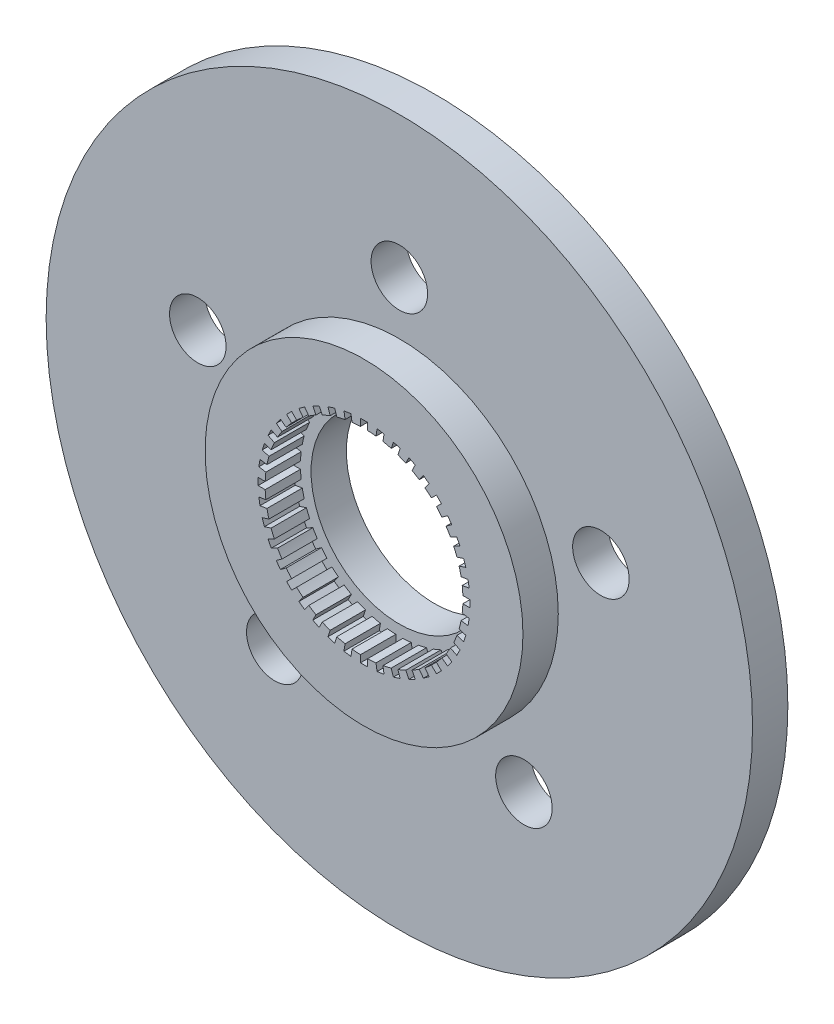
from build123d import *

# Parameters (mm, degrees)
SKETCH_1_R      = 100
SKETCH_1_R_2    = 25
SKETCH_1_R_3    = 8
EXTRUDE_1_DEPTH = 10
EXTRUDE_START   = -10
SKETCH_2_R      = 45
EXTRUDE_2_DEPTH = 20


with BuildPart() as part:
    # 草图1 → 凸台-拉伸1 (new body)
    with BuildSketch(Plane.XY):
        Circle(SKETCH_1_R)
        Circle(SKETCH_1_R_2, mode=Mode.SUBTRACT)
        with Locations((0, 60)):
            Circle(SKETCH_1_R_3, mode=Mode.SUBTRACT)
        with Locations((57.063390978, 18.541019663)):
            Circle(SKETCH_1_R_3, mode=Mode.SUBTRACT)
        with Locations((35.267115138, -48.541019662)):
            Circle(SKETCH_1_R_3, mode=Mode.SUBTRACT)
        with Locations((-35.267115138, -48.541019663)):
            Circle(SKETCH_1_R_3, mode=Mode.SUBTRACT)
        with Locations((-57.063390978, 18.541019662)):
            Circle(SKETCH_1_R_3, mode=Mode.SUBTRACT)
    extrude(amount=EXTRUDE_1_DEPTH)

    # 草图2 → 凸台-拉伸2 (add)
    with BuildSketch(Plane.XY.offset(10).offset(EXTRUDE_START)):
        Circle(SKETCH_2_R)
        with BuildLine():
            Line((3.389682317, 27.794065082), (3.702737645, 29.770618635))
            Line((3.702737645, 29.770618635), (5.678114326, 29.457749705))
            Line((5.678114326, 29.457749705), (5.365058998, 27.481196152))
            ThreePointArc((5.365058998, 27.481196152), (6.536470188, 27.226357771), (7.695899405, 26.92161088))
            Line((7.695899405, 26.92161088), (8.3143016, 28.824857136))
            Line((8.3143016, 28.824857136), (10.216414633, 28.206823147))
            Line((10.216414633, 28.206823147), (9.598012437, 26.303576891))
            ThreePointArc((9.598012437, 26.303576891), (10.715136106, 25.86862691), (11.812617909, 25.386257269))
            Line((11.812617909, 25.386257269), (12.721139857, 27.169331989))
            Line((12.721139857, 27.169331989), (14.503152905, 26.26135099))
            Line((14.503152905, 26.26135099), (13.594630957, 24.47827627))
            ThreePointArc((13.594630957, 24.47827627), (14.629959812, 23.873924602), (15.638470555, 23.225809753))
            Line((15.638470555, 23.225809753), (16.814741431, 24.844807719))
            Line((16.814741431, 24.844807719), (18.43277542, 23.669237215))
            Line((18.43277542, 23.669237215), (17.256504544, 22.050239248))
            ThreePointArc((17.256504544, 22.050239248), (18.184545353, 21.291367037), (19.079252156, 20.493465719))
            Line((19.079252156, 20.493465719), (20.494308266, 21.908521828))
            Line((20.494308266, 21.908521828), (21.908521828, 20.494308266))
            Line((21.908521828, 20.494308266), (20.493465719, 19.079252156))
            ThreePointArc((20.493465719, 19.079252156), (21.291367037, 18.184545353), (22.050239248, 17.256504544))
            Line((22.050239248, 17.256504544), (23.669237215, 18.43277542))
            Line((23.669237215, 18.43277542), (24.844807719, 16.814741431))
            Line((24.844807719, 16.814741431), (23.225809753, 15.638470555))
            ThreePointArc((23.225809753, 15.638470555), (23.873924602, 14.629959812), (24.47827627, 13.594630957))
            Line((24.47827627, 13.594630957), (26.26135099, 14.503152905))
            Line((26.26135099, 14.503152905), (27.169331989, 12.721139857))
            Line((27.169331989, 12.721139857), (25.386257269, 11.812617909))
            ThreePointArc((25.386257269, 11.812617909), (25.86862691, 10.715136106), (26.303576891, 9.598012437))
            Line((26.303576891, 9.598012437), (28.206823147, 10.216414633))
            Line((28.206823147, 10.216414633), (28.824857136, 8.3143016))
            Line((28.824857136, 8.3143016), (26.92161088, 7.695899405))
            ThreePointArc((26.92161088, 7.695899405), (27.226357771, 6.536470188), (27.481196152, 5.365058998))
            Line((27.481196152, 5.365058998), (29.457749705, 5.678114326))
            Line((29.457749705, 5.678114326), (29.770618635, 3.702737645))
            Line((29.770618635, 3.702737645), (27.794065082, 3.389682317))
            ThreePointArc((27.794065082, 3.389682317), (27.913685345, 2.19685468), (27.982137159, 1))
            Line((27.982137159, 1), (29.983328701, 1))
            Line((29.983328701, 1), (29.983328701, -1))
            Line((29.983328701, -1), (27.982137159, -1))
            ThreePointArc((27.982137159, -1), (27.913685345, -2.19685468), (27.794065082, -3.389682317))
            Line((27.794065082, -3.389682317), (29.770618635, -3.702737645))
            Line((29.770618635, -3.702737645), (29.457749705, -5.678114326))
            Line((29.457749705, -5.678114326), (27.481196152, -5.365058998))
            ThreePointArc((27.481196152, -5.365058998), (27.226357771, -6.536470188), (26.92161088, -7.695899405))
            Line((26.92161088, -7.695899405), (28.824857136, -8.3143016))
            Line((28.824857136, -8.3143016), (28.206823147, -10.216414633))
            Line((28.206823147, -10.216414633), (26.303576891, -9.598012437))
            ThreePointArc((26.303576891, -9.598012437), (25.86862691, -10.715136106), (25.386257269, -11.812617909))
            Line((25.386257269, -11.812617909), (27.169331989, -12.721139857))
            Line((27.169331989, -12.721139857), (26.26135099, -14.503152905))
            Line((26.26135099, -14.503152905), (24.47827627, -13.594630957))
            ThreePointArc((24.47827627, -13.594630957), (23.873924602, -14.629959812), (23.225809753, -15.638470555))
            Line((23.225809753, -15.638470555), (24.844807719, -16.814741431))
            Line((24.844807719, -16.814741431), (23.669237215, -18.43277542))
            Line((23.669237215, -18.43277542), (22.050239248, -17.256504544))
            ThreePointArc((22.050239248, -17.256504544), (21.291367037, -18.184545353), (20.493465719, -19.079252156))
            Line((20.493465719, -19.079252156), (21.908521828, -20.494308266))
            Line((21.908521828, -20.494308266), (20.494308266, -21.908521828))
            Line((20.494308266, -21.908521828), (19.079252156, -20.493465719))
            ThreePointArc((19.079252156, -20.493465719), (18.184545353, -21.291367037), (17.256504544, -22.050239248))
            Line((17.256504544, -22.050239248), (18.43277542, -23.669237215))
            Line((18.43277542, -23.669237215), (16.814741431, -24.844807719))
            Line((16.814741431, -24.844807719), (15.638470555, -23.225809753))
            ThreePointArc((15.638470555, -23.225809753), (14.629959812, -23.873924602), (13.594630957, -24.47827627))
            Line((13.594630957, -24.47827627), (14.503152905, -26.26135099))
            Line((14.503152905, -26.26135099), (12.721139857, -27.169331989))
            Line((12.721139857, -27.169331989), (11.812617909, -25.386257269))
            ThreePointArc((11.812617909, -25.386257269), (10.715136106, -25.86862691), (9.598012437, -26.303576891))
            Line((9.598012437, -26.303576891), (10.216414633, -28.206823147))
            Line((10.216414633, -28.206823147), (8.3143016, -28.824857136))
            Line((8.3143016, -28.824857136), (7.695899405, -26.92161088))
            ThreePointArc((7.695899405, -26.92161088), (6.536470188, -27.226357771), (5.365058998, -27.481196152))
            Line((5.365058998, -27.481196152), (5.678114326, -29.457749705))
            Line((5.678114326, -29.457749705), (3.702737645, -29.770618635))
            Line((3.702737645, -29.770618635), (3.389682317, -27.794065082))
            ThreePointArc((3.389682317, -27.794065082), (2.19685468, -27.913685345), (1, -27.982137159))
            Line((1, -27.982137159), (1, -29.983328701))
            Line((1, -29.983328701), (-1, -29.983328701))
            Line((-1, -29.983328701), (-1, -27.982137159))
            ThreePointArc((-1, -27.982137159), (-2.19685468, -27.913685345), (-3.389682317, -27.794065082))
            Line((-3.389682317, -27.794065082), (-3.702737645, -29.770618635))
            Line((-3.702737645, -29.770618635), (-5.678114326, -29.457749705))
            Line((-5.678114326, -29.457749705), (-5.365058998, -27.481196152))
            ThreePointArc((-5.365058998, -27.481196152), (-6.536470188, -27.226357771), (-7.695899405, -26.92161088))
            Line((-7.695899405, -26.92161088), (-8.3143016, -28.824857136))
            Line((-8.3143016, -28.824857136), (-10.216414633, -28.206823147))
            Line((-10.216414633, -28.206823147), (-9.598012437, -26.303576891))
            ThreePointArc((-9.598012437, -26.303576891), (-10.715136106, -25.86862691), (-11.812617909, -25.386257269))
            Line((-11.812617909, -25.386257269), (-12.721139857, -27.169331989))
            Line((-12.721139857, -27.169331989), (-14.503152905, -26.26135099))
            Line((-14.503152905, -26.26135099), (-13.594630957, -24.47827627))
            ThreePointArc((-13.594630957, -24.47827627), (-14.629959812, -23.873924602), (-15.638470555, -23.225809753))
            Line((-15.638470555, -23.225809753), (-16.814741431, -24.844807719))
            Line((-16.814741431, -24.844807719), (-18.43277542, -23.669237215))
            Line((-18.43277542, -23.669237215), (-17.256504544, -22.050239248))
            ThreePointArc((-17.256504544, -22.050239248), (-18.184545353, -21.291367037), (-19.079252156, -20.493465719))
            Line((-19.079252156, -20.493465719), (-20.494308266, -21.908521828))
            Line((-20.494308266, -21.908521828), (-21.908521828, -20.494308266))
            Line((-21.908521828, -20.494308266), (-20.493465719, -19.079252156))
            ThreePointArc((-20.493465719, -19.079252156), (-21.291367037, -18.184545353), (-22.050239248, -17.256504544))
            Line((-22.050239248, -17.256504544), (-23.669237215, -18.43277542))
            Line((-23.669237215, -18.43277542), (-24.844807719, -16.814741431))
            Line((-24.844807719, -16.814741431), (-23.225809753, -15.638470555))
            ThreePointArc((-23.225809753, -15.638470555), (-23.873924602, -14.629959812), (-24.47827627, -13.594630957))
            Line((-24.47827627, -13.594630957), (-26.26135099, -14.503152905))
            Line((-26.26135099, -14.503152905), (-27.169331989, -12.721139857))
            Line((-27.169331989, -12.721139857), (-25.386257269, -11.812617909))
            ThreePointArc((-25.386257269, -11.812617909), (-25.86862691, -10.715136106), (-26.303576891, -9.598012437))
            Line((-26.303576891, -9.598012437), (-28.206823147, -10.216414633))
            Line((-28.206823147, -10.216414633), (-28.824857136, -8.3143016))
            Line((-28.824857136, -8.3143016), (-26.92161088, -7.695899405))
            ThreePointArc((-26.92161088, -7.695899405), (-27.226357771, -6.536470188), (-27.481196152, -5.365058998))
            Line((-27.481196152, -5.365058998), (-29.457749705, -5.678114326))
            Line((-29.457749705, -5.678114326), (-29.770618635, -3.702737645))
            Line((-29.770618635, -3.702737645), (-27.794065082, -3.389682317))
            ThreePointArc((-27.794065082, -3.389682317), (-27.913685345, -2.19685468), (-27.982137159, -1))
            Line((-27.982137159, -1), (-29.983328701, -1))
            Line((-29.983328701, -1), (-29.983328701, 1))
            Line((-29.983328701, 1), (-27.982137159, 1))
            ThreePointArc((-27.982137159, 1), (-27.913685345, 2.19685468), (-27.794065082, 3.389682317))
            Line((-27.794065082, 3.389682317), (-29.770618635, 3.702737645))
            Line((-29.770618635, 3.702737645), (-29.457749705, 5.678114326))
            Line((-29.457749705, 5.678114326), (-27.481196152, 5.365058998))
            ThreePointArc((-27.481196152, 5.365058998), (-27.226357771, 6.536470188), (-26.92161088, 7.695899405))
            Line((-26.92161088, 7.695899405), (-28.824857136, 8.3143016))
            Line((-28.824857136, 8.3143016), (-28.206823147, 10.216414633))
            Line((-28.206823147, 10.216414633), (-26.303576891, 9.598012437))
            ThreePointArc((-26.303576891, 9.598012437), (-25.86862691, 10.715136106), (-25.386257269, 11.812617909))
            Line((-25.386257269, 11.812617909), (-27.169331989, 12.721139857))
            Line((-27.169331989, 12.721139857), (-26.26135099, 14.503152905))
            Line((-26.26135099, 14.503152905), (-24.47827627, 13.594630957))
            ThreePointArc((-24.47827627, 13.594630957), (-23.873924602, 14.629959812), (-23.225809753, 15.638470555))
            Line((-23.225809753, 15.638470555), (-24.844807719, 16.814741431))
            Line((-24.844807719, 16.814741431), (-23.669237215, 18.43277542))
            Line((-23.669237215, 18.43277542), (-22.050239248, 17.256504544))
            ThreePointArc((-22.050239248, 17.256504544), (-21.291367037, 18.184545353), (-20.493465719, 19.079252156))
            Line((-20.493465719, 19.079252156), (-21.908521828, 20.494308266))
            Line((-21.908521828, 20.494308266), (-20.494308266, 21.908521828))
            Line((-20.494308266, 21.908521828), (-19.079252156, 20.493465719))
            ThreePointArc((-19.079252156, 20.493465719), (-18.184545353, 21.291367037), (-17.256504544, 22.050239248))
            Line((-17.256504544, 22.050239248), (-18.43277542, 23.669237215))
            Line((-18.43277542, 23.669237215), (-16.814741431, 24.844807719))
            Line((-16.814741431, 24.844807719), (-15.638470555, 23.225809753))
            ThreePointArc((-15.638470555, 23.225809753), (-14.629959812, 23.873924602), (-13.594630957, 24.47827627))
            Line((-13.594630957, 24.47827627), (-14.503152905, 26.26135099))
            Line((-14.503152905, 26.26135099), (-12.721139857, 27.169331989))
            Line((-12.721139857, 27.169331989), (-11.812617909, 25.386257269))
            ThreePointArc((-11.812617909, 25.386257269), (-10.715136106, 25.86862691), (-9.598012437, 26.303576891))
            Line((-9.598012437, 26.303576891), (-10.216414633, 28.206823147))
            Line((-10.216414633, 28.206823147), (-8.3143016, 28.824857136))
            Line((-8.3143016, 28.824857136), (-7.695899405, 26.92161088))
            ThreePointArc((-7.695899405, 26.92161088), (-6.536470188, 27.226357771), (-5.365058998, 27.481196152))
            Line((-5.365058998, 27.481196152), (-5.678114326, 29.457749705))
            Line((-5.678114326, 29.457749705), (-3.702737645, 29.770618635))
            Line((-3.702737645, 29.770618635), (-3.389682317, 27.794065082))
            ThreePointArc((-3.389682317, 27.794065082), (-2.19685468, 27.913685345), (-1, 27.982137159))
            Line((-1, 27.982137159), (-1, 29.983328701))
            Line((-1, 29.983328701), (1, 29.983328701))
            Line((1, 29.983328701), (1, 27.982137159))
            ThreePointArc((1, 27.982137159), (2.19685468, 27.913685345), (3.389682317, 27.794065082))
        make_face(mode=Mode.SUBTRACT)
    extrude(amount=EXTRUDE_2_DEPTH)


solid = part.part
